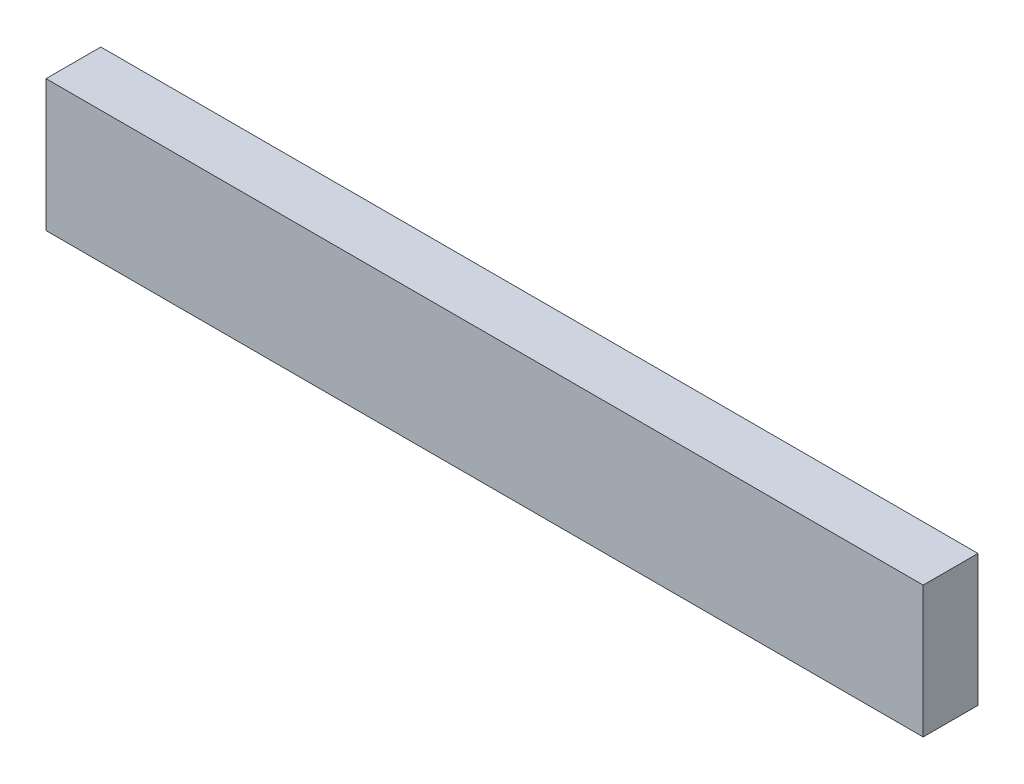
SolidWorks part; units mm, degrees
ref_plane "前视基准面" through (0, 0, 0) normal (0, 0, 1) x (1, 0, 0)
ref_plane "上视基准面" through (0, 0, 0) normal (0, 1, 0) x (1, 0, 0)
ref_plane "右视基准面" through (0, 0, 0) normal (1, 0, 0) x (0, 0, -1)
sketch "草图1" plane through (0, 0, 0) normal (0, 0, 1) x (1, 0, 0)
  line L1 (-40.6762, 113.7661) -> (759.3238, 113.7661)
  line L2 (-40.6762, 113.7661) -> (-40.6762, -6.2339)
  line L3 (-40.6762, -6.2339) -> (759.3238, -6.2339)
  line L4 (759.3238, 113.7661) -> (759.3238, -6.2339)
extrude "凸台-拉伸1" add sketch "草图1" along normal blind 50
